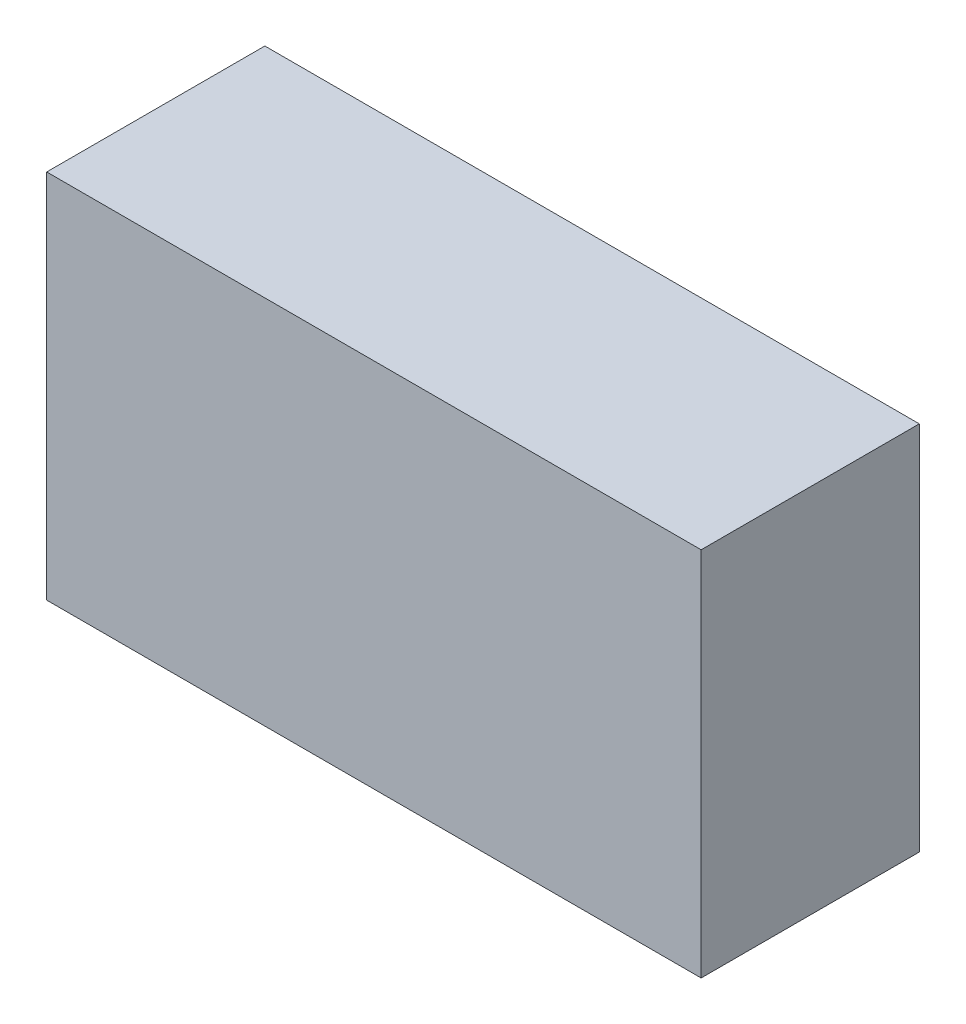
from build123d import *

# Parameters (mm, degrees)
SKETCH_1_W      = 300
SKETCH_1_H      = 170
EXTRUDE_1_DEPTH = 50


with BuildPart() as part:
    # 草图1 → 凸台-拉伸1 (new, symmetric)
    with BuildSketch(Plane.XY):
        Rectangle(SKETCH_1_W, SKETCH_1_H)
    extrude(amount=EXTRUDE_1_DEPTH, both=True)


solid = part.part
